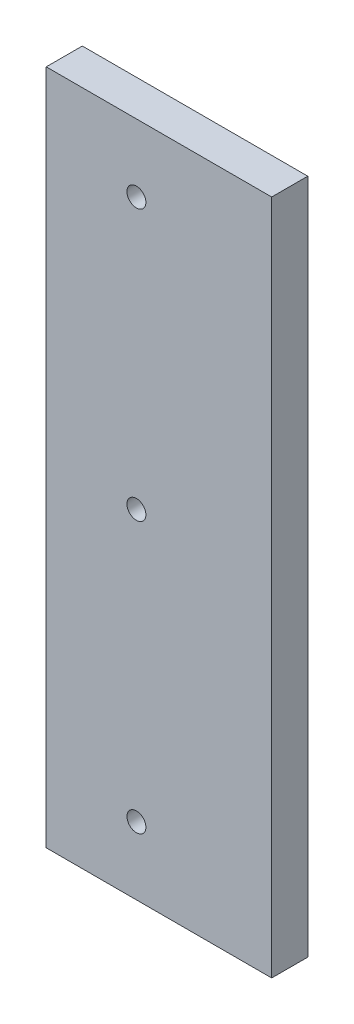
SolidWorks part; units mm, degrees
material "Q235B"
ref_plane "Front Plane" through (0, 0, 0) normal (0, 0, 1) x (1, 0, 0)
ref_plane "Top Plane" through (0, 0, 0) normal (0, 1, 0) x (1, 0, 0)
ref_plane "Right Plane" through (0, 0, 0) normal (1, 0, 0) x (0, 0, -1)
sketch "Sketch1" plane through (0, 0, 0) normal (0, 0, 1) x (1, 0, 0)
  line L1 (25, -75) -> (-25, -75)
  line L2 (25, -75) -> (25, 75)
  line L3 (25, 75) -> (-25, 75)
  line L4 (-25, -75) -> (-25, 75)
  line L5 (25, -75) -> (-25, 75) construction
  line L6 (25, 75) -> (-25, -75) construction
  point P0 (0, 0)
  dimension "D1" = 150
  dimension "D2" = 50
extrude "Boss-Extrude1" add sketch "Sketch1" along normal mid plane 8
hole_wizard "M5 Tapped Hole1" positions "Sketch2" profile "Sketch3" tap size "M5" standard "GB" end condition up to next
sketch "Sketch2" plane through (0, 0, 4) normal (0, 0, 1) x (1, 0, 0)
  line L0 (0, 75) -> (0, 0) construction
  line L1 (25, 75) -> (-25, 75) construction
  line L2 (0, 0) -> (-25, 0) construction
  line L3 (-25, 75) -> (-25, -75) construction
  line L4 (25, -75) -> (25, 75) construction
  point P0 (-5, 60)
  point P15 (-5, -60)
  point P16 (-5, 0)
  dimension "D1" = 30
  dimension "D2" = 120
sketch "Sketch3" plane through (-5, 60, 4) normal (1, 0, 0) x (0, -1, 0)
  line L0 (0, 0) -> (0, 8)
  line L1 (0, 8) -> (2.1, 8)
  line L2 (2.1, 8) -> (2.1, 0)
  line L5 (2.1, 0) -> (0, 0)
  line L11 (0, -6.35) -> (0, 107.95) construction
  dimension "通孔螺纹孔钻头直径" = 4.2
  dimension "通孔螺纹孔钻头深度" = 8
cosmetic thread "Hole Cosmetic Thread1" parameters "D2"=5
cosmetic thread "Hole Cosmetic Thread2" parameters "D2"=5
cosmetic thread "Hole Cosmetic Thread3" parameters "D2"=5
chamfer "Chamfer1" [suppressed] distance 10 angle 45
